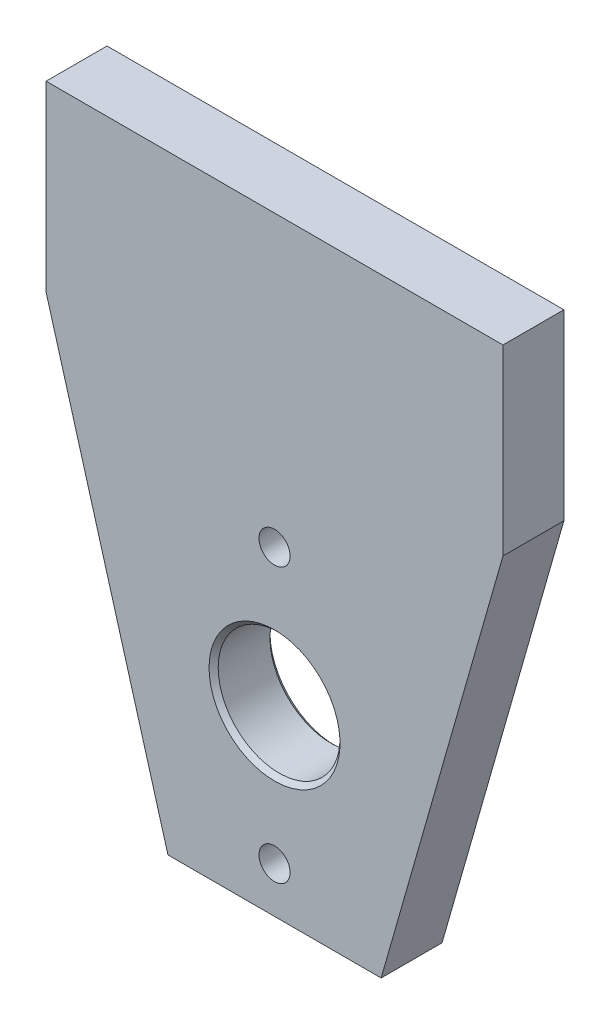
SolidWorks part; units mm, degrees
material "1023 碳钢板 (SS)"
ref_plane "Front Plane" through (0, 0, 0) normal (0, 0, 1) x (1, 0, 0)
ref_plane "Top Plane" through (0, 0, 0) normal (0, 1, 0) x (1, 0, 0)
ref_plane "Right Plane" through (0, 0, 0) normal (1, 0, 0) x (0, 0, -1)
sketch "Sketch1" plane through (0, 0, 0) normal (0, 0, 1) x (1, 0, 0)
  line L0 (0, 0) -> (150, 0)
  line L1 (150, 0) -> (150, -60)
  line L2 (150, -60) -> (110, -200)
  line L3 (110, -200) -> (40, -200)
  line L4 (40, -200) -> (0, -60)
  line L5 (0, -60) -> (0, 0)
  circle A0 centre (75, -140) radius 20
  dimension "D5" = 40
  dimension "D1" = 200
  dimension "D2" = 70
  dimension "D3" = 60
  dimension "D4" = 150
  dimension "D6" = 60
extrude "Boss-Extrude1" add sketch "Sketch1" along normal blind 20
sketch "Sketch2" plane through (0, 0, 20) normal (0, 0, 1) x (1, 0, 0)
  circle A0 centre (75, -95) radius 7.4206
  circle A1 centre (75, -185) radius 9.6209
  circle A2 centre (75, -140) radius 20 construction
  dimension "D2" = 45
  dimension "D1" = 90
hole_wizard "M12 Tapped Hole1" positions "Sketch3" profile "Sketch4" tap size "M12" standard "ISO"
sketch "Sketch3" plane through (0, 0, 20) normal (0, 0, 1) x (1, 0, 0)
  point P0 (75, -95)
  point P3 (75, -185)
sketch "Sketch4" plane through (75, -95, 20) normal (1, 0, 0) x (0, -1, 0)
  line L0 (0, 0) -> (0, 32.3144)
  line L1 (0, 32.3144) -> (5.1, 29.25)
  line L2 (5.1, 29.25) -> (5.1, 0)
  line L5 (5.1, 0) -> (0, 0)
  line L10 (0, 32.3144) -> (-5.1, 29.25) construction
  line L11 (0, -6.35) -> (0, 107.95) construction
  dimension "螺纹孔钻头直径" = 10.2
  dimension "螺纹孔钻头深度" = 29.25
  dimension "导头角度" = 118
cosmetic thread "Hole Thread Line1"
cosmetic thread "Hole Thread Line2"
chamfer "Chamfer1" distance 1.5 angle 45 2 edges at (95, -140, 0) (95, -140, 20)
